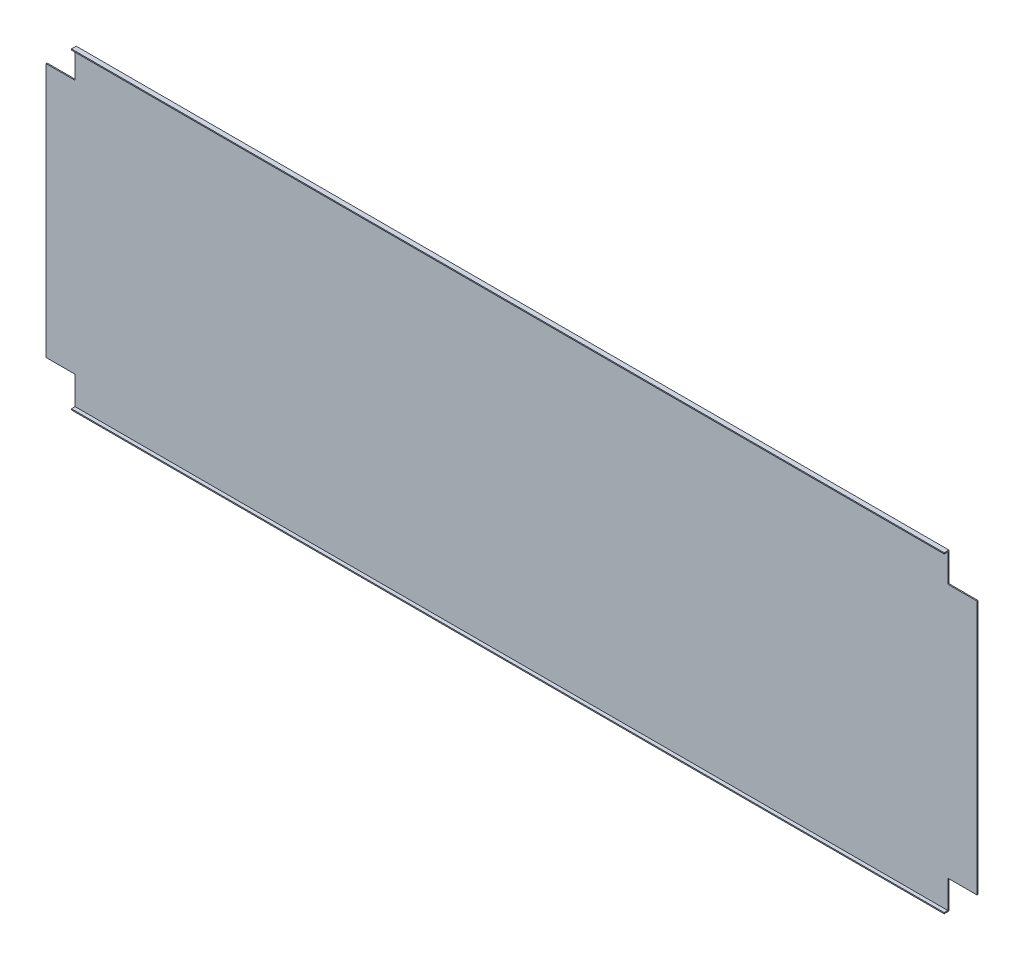
SolidWorks part; units mm, degrees
ref_plane "Front Plane" through (0, 0, 0) normal (0, 0, 1) x (1, 0, 0)
ref_plane "Top Plane" through (0, 0, 0) normal (0, 1, 0) x (1, 0, 0)
ref_plane "Right Plane" through (0, 0, 0) normal (1, 0, 0) x (0, 0, -1)
sketch "Sketch1" plane through (0, 0, 0) normal (0, 0, 1) x (1, 0, 0)
  line L1 (40, 0) -> (1240, 0)
  line L2 (0, 40) -> (0, 390)
  line L3 (40, 430) -> (1240, 430)
  line L4 (1280, 40) -> (1280, 390)
  line L7 (0, 390) -> (40, 390)
  line L8 (40, 430) -> (40, 390)
  line L11 (0, 40) -> (40, 40)
  line L12 (40, 0) -> (40, 40)
  line L15 (1280, 40) -> (1240, 40)
  line L16 (1240, 0) -> (1240, 40)
  line L19 (1280, 390) -> (1240, 390)
  line L20 (1240, 430) -> (1240, 390)
extrude "Boss-Extrude1" add sketch "Sketch1" along normal blind 1.5
sketch "Sketch2" plane through (0, 0, 1.5) normal (0, 0, 1) x (1, 0, 0)
  line L1 (40, 430) -> (1240, 430)
  line L2 (40, 430) -> (40, 428.5)
  line L3 (40, 428.5) -> (1240, 428.5)
  line L4 (1240, 430) -> (1240, 428.5)
  line L9 (40, 0) -> (1240, 0)
  line L10 (40, 0) -> (40, 1.5)
  line L11 (40, 1.5) -> (1240, 1.5)
  line L12 (1240, 0) -> (1240, 1.5)
extrude "Boss-Extrude2" add sketch "Sketch2" along normal blind 5
